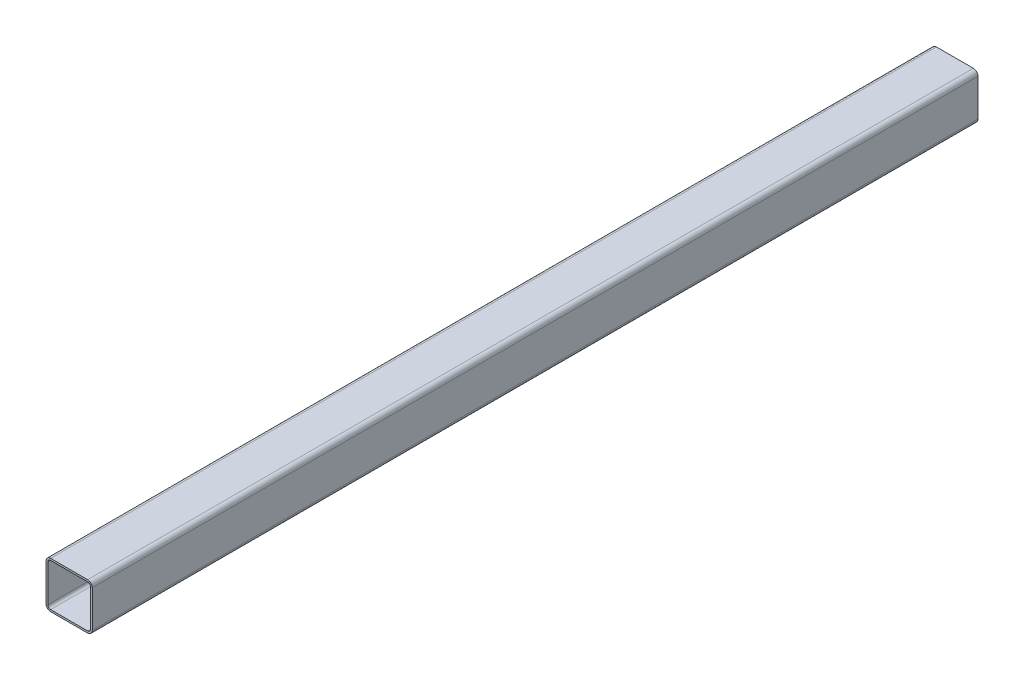
SolidWorks part; units mm, degrees
ref_plane "Front Plane" through (0, 0, 0) normal (0, 0, 1) x (1, 0, 0)
ref_plane "Top Plane" through (0, 0, 0) normal (0, 1, 0) x (1, 0, 0)
ref_plane "Right Plane" through (0, 0, 0) normal (1, 0, 0) x (0, 0, -1)
other "Configuration Table"
sketch "Sketch1" plane through (0, 0, 0) normal (0, 0, 1) x (1, 0, 0)
  line L0 (-92, 80) -> (-92, -80)
  line L1 (-80, 100) -> (80, 100)
  line L2 (-100, 80) -> (-100, -80)
  line L3 (-80, -100) -> (80, -100)
  line L4 (100, 80) -> (100, -80)
  line L5 (-100, 100) -> (100, -100) construction
  line L6 (-100, -100) -> (100, 100) construction
  line L7 (-80, -92) -> (80, -92)
  line L8 (92, 80) -> (92, -80)
  line L9 (-80, 92) -> (80, 92)
  arc A0 (-100, -80) -> (-80, -100) centre (-80, -80) ccw
  arc A1 (80, -100) -> (100, -80) centre (80, -80) ccw
  arc A2 (80, 100) -> (100, 80) centre (80, 80) cw
  arc A3 (-80, 100) -> (-100, 80) centre (-80, 80) ccw
  arc A4 (-92, -80) -> (-80, -92) centre (-80, -80) ccw
  arc A5 (80, -92) -> (92, -80) centre (80, -80) ccw
  arc A6 (80, 92) -> (92, 80) centre (80, 80) cw
  arc A7 (-80, 92) -> (-92, 80) centre (-80, 80) ccw
  point P0 (0, 0)
  dimension "D3" = 20
  dimension "D1" = 200
  dimension "D2" = 200
  dimension "D4" = 8
extrude "Boss-Extrude1" add sketch "Sketch1" along normal blind 3830
